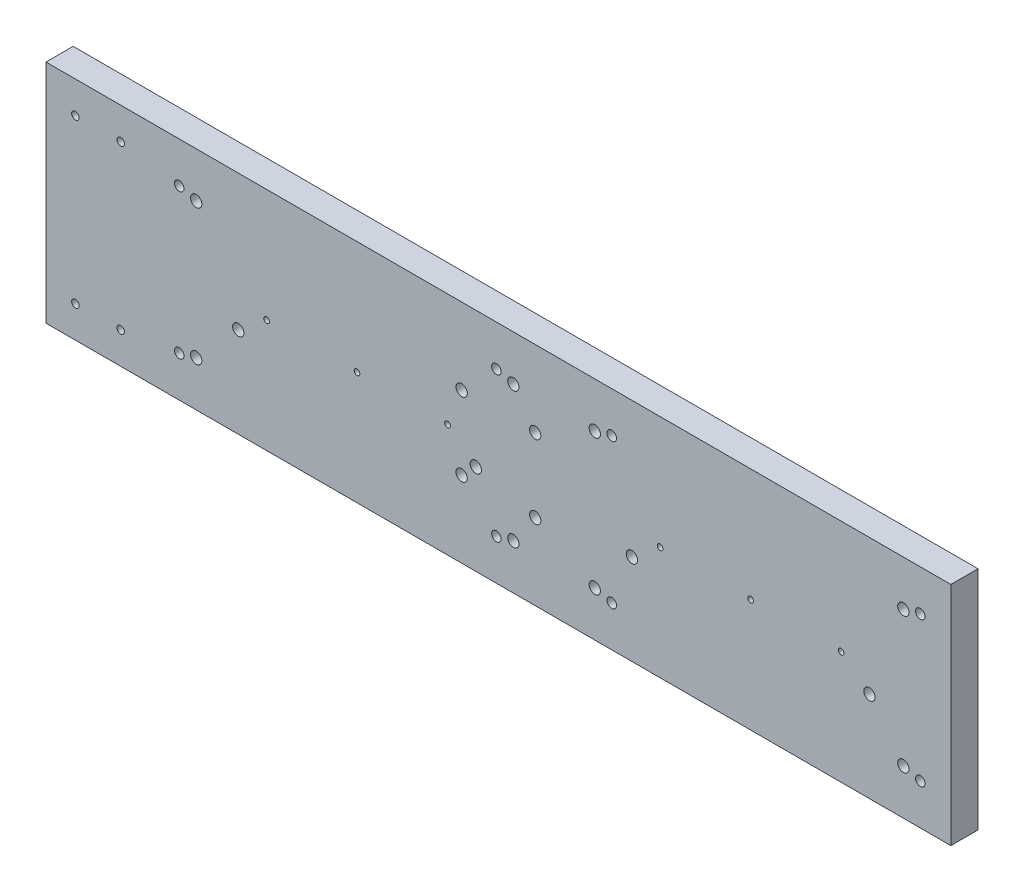
from build123d import *

# Parameters (mm, degrees)
SKETCH1_W           = 400
SKETCH1_H           = 100
BOSS_EXTRUDE1_DEPTH = 12
M4_TAPPED_HOLE1_D   = 3.3
M5_TAPPED_HOLE1_D   = 4.2
SKETCH6_R           = 2.5
CUT_EXTRUDE1_DEPTH  = 413.485151248
M6_TAPPED_HOLE1_D   = 5
M3_TAPPED_HOLE1_D   = 2.5


with BuildPart() as part:
    # Sketch1 → Boss-Extrude1 (new body)
    with BuildSketch(Plane.XY):
        with Locations((200, 50)):
            Rectangle(SKETCH1_W, SKETCH1_H)
    extrude(amount=BOSS_EXTRUDE1_DEPTH)

    # M4 Tapped Hole1 (through all)
    with Locations(Plane.XY.offset(12)):
        with Locations((13, 14), (13, 86), (33, 86), (33, 14)):
            Hole(M4_TAPPED_HOLE1_D / 2)

    # M5 Tapped Hole1 (through all)
    with Locations(Plane.XY.offset(12)):
        with Locations((58.9, 82), (58.9, 18), (199.1, 82), (199.1, 18), (250.1, 18), (250.1, 82), (386.5, 82), (386.5, 18)):
            Hole(M5_TAPPED_HOLE1_D / 2)

    # Sketch6 → Cut-Extrude1 (cut, through all)
    with BuildSketch(Plane.XY.offset(12)):
        with Locations((66.4, 80)):
            Circle(SKETCH6_R)
        with Locations((66.4, 20)):
            Circle(SKETCH6_R)
        with Locations((206.6, 80)):
            Circle(SKETCH6_R)
        with Locations((206.6, 20)):
            Circle(SKETCH6_R)
        with Locations((242.6, 20)):
            Circle(SKETCH6_R)
        with Locations((242.6, 80)):
            Circle(SKETCH6_R)
        with Locations((379, 80)):
            Circle(SKETCH6_R)
        with Locations((379, 20)):
            Circle(SKETCH6_R)
        with Locations((85, 40)):
            Circle(SKETCH6_R)
        with Locations((190, 40)):
            Circle(SKETCH6_R)
        with Locations((259, 40)):
            Circle(SKETCH6_R)
        with Locations((364, 40)):
            Circle(SKETCH6_R)
    extrude(amount=-CUT_EXTRUDE1_DEPTH, mode=Mode.SUBTRACT)

    # M6 Tapped Hole1 (through all)
    with Locations(Plane.XY.offset(12)):
        with Locations((183.736544033, 66.263455967), (216.263455967, 66.263455967), (216.263455967, 33.736544033), (183.736544033, 33.736544033)):
            Hole(M6_TAPPED_HOLE1_D / 2)

    # M3 Tapped Hole1 (through all)
    with Locations(Plane.XY.offset(12)):
        with Locations((97.5, 50), (137.5, 50), (177.5, 50), (271.5, 50), (311.5, 50), (351.5, 50)):
            Hole(M3_TAPPED_HOLE1_D / 2)


solid = part.part
